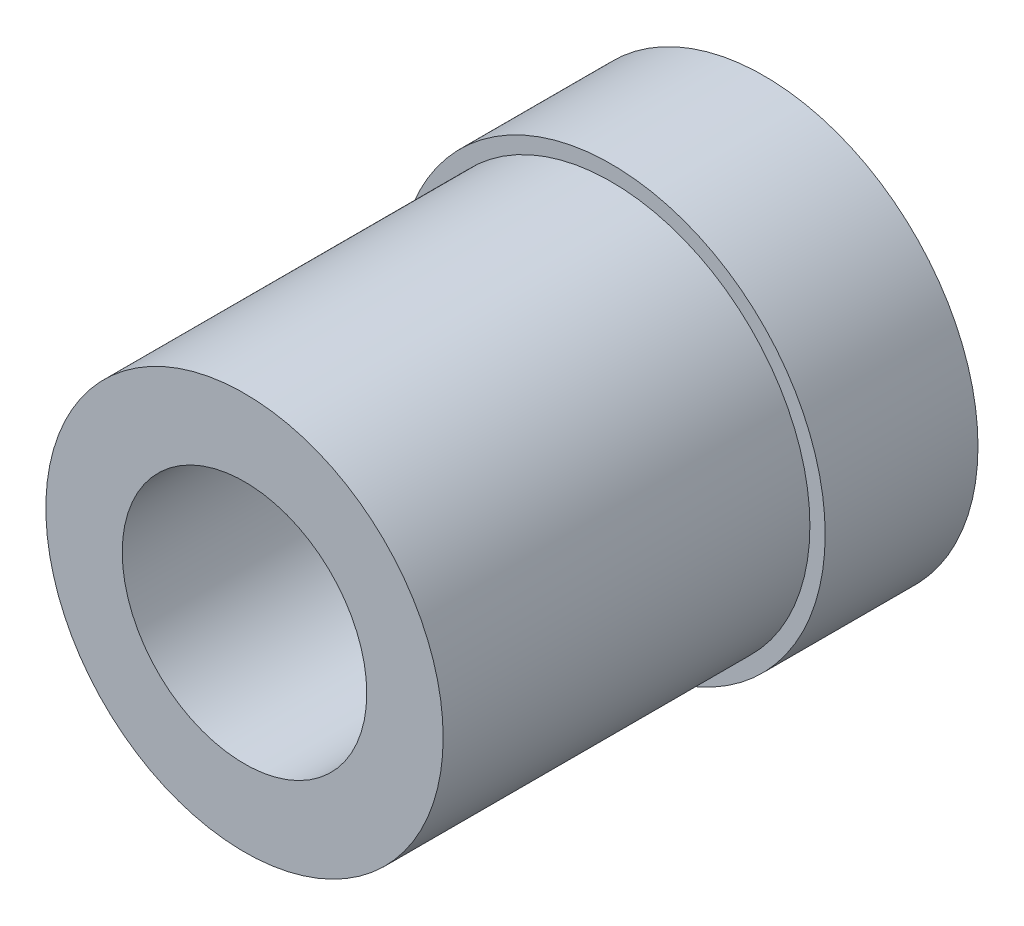
from build123d import *

# Parameters (mm, degrees)
SKETCH1_R           = 7
SKETCH1_R_2         = 4
BOSS_EXTRUDE1_DEPTH = 5
SKETCH2_R           = 6.5
SKETCH2_R_2         = 4
BOSS_EXTRUDE2_DEPTH = 12


with BuildPart() as part:
    # Sketch1 → Boss-Extrude1 (new body)
    with BuildSketch(Plane.XY):
        Circle(SKETCH1_R)
        Circle(SKETCH1_R_2, mode=Mode.SUBTRACT)
    extrude(amount=BOSS_EXTRUDE1_DEPTH)

    # Sketch2 → Boss-Extrude2 (add)
    with BuildSketch(Plane.XY.offset(5)):
        Circle(SKETCH2_R)
        Circle(SKETCH2_R_2, mode=Mode.SUBTRACT)
    extrude(amount=BOSS_EXTRUDE2_DEPTH)


solid = part.part
